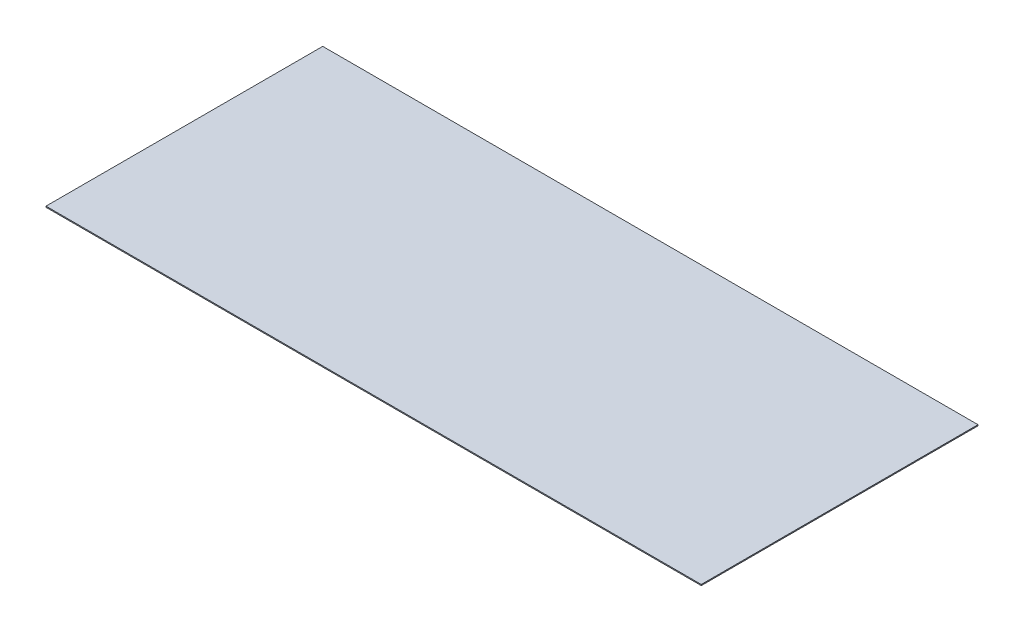
SolidWorks part; units mm, degrees
ref_plane "Front Plane" through (0, 0, 0) normal (0, 0, 1) x (1, 0, 0)
ref_plane "Top Plane" through (0, 0, 0) normal (0, 1, 0) x (1, 0, 0)
ref_plane "Right Plane" through (0, 0, 0) normal (1, 0, 0) x (0, 0, -1)
sketch "Sketch 1" plane through (0, 0, 0) normal (0, 1, 0) x (1, 0, 0)
  line L1 (-2510, -1060) -> (2510, -1060)
  line L2 (-2510, -1060) -> (-2510, 1060)
  line L3 (-2510, 1060) -> (2510, 1060)
  line L4 (2510, -1060) -> (2510, 1060)
  line L5 (-2510, -1060) -> (2510, 1060) construction
  line L6 (-2510, 1060) -> (2510, -1060) construction
  point P0 (0, 0)
  dimension "D1" = 5020
  dimension "D2" = 2120
extrude "Boss-Extrude 1" add sketch "Sketch 1" along normal blind 8
